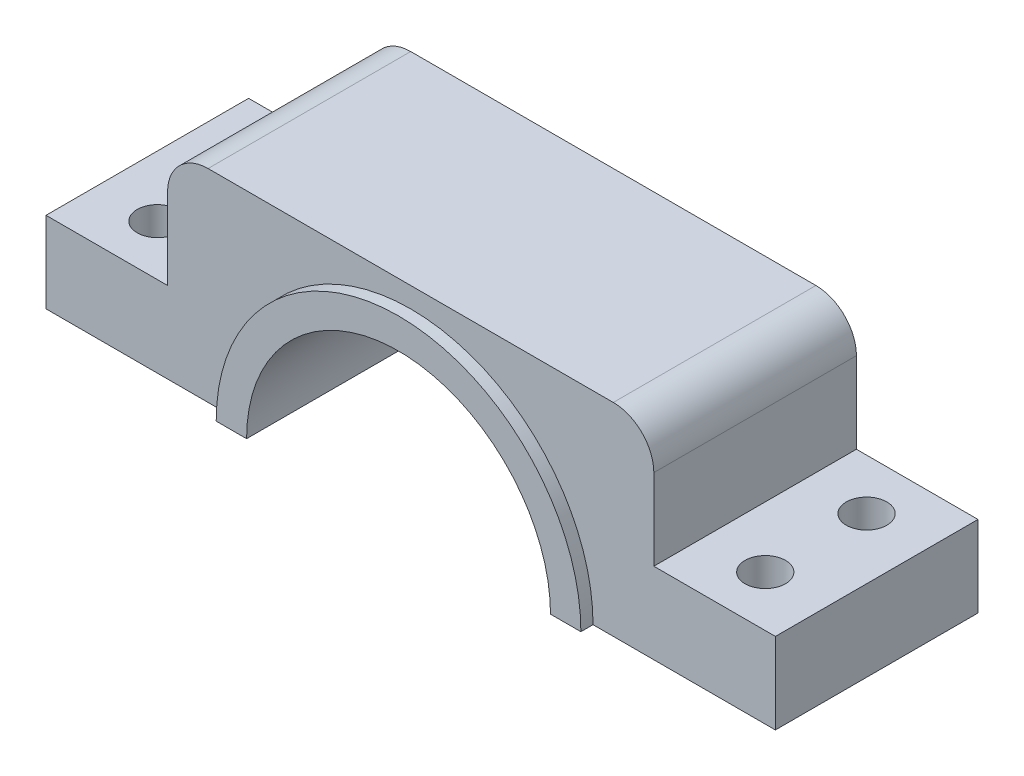
from build123d import *

# Parameters (mm, degrees)
SKETCH_2_W          = 120
SKETCH_2_H          = 50
EXTRUDE_1_DEPTH     = 50
SKETCH_3_R          = 37.5
CUT_EXTRUDE_1_DEPTH = 139
FILLET_1_R          = 10
SKETCH_4_W          = 30
SKETCH_4_H          = 50
EXTRUDE_2_DEPTH     = 20
EXTRUDE_START       = 3
EXTRUDE_3_DEPTH     = 3
SKETCH_6_R          = 5
CUT_EXTRUDE_2_DEPTH = 38


with BuildPart() as part:
    # 草图2 → 凸台-拉伸1 (new body)
    with BuildSketch(Plane(origin=(0, 0, 0), x_dir=(1, 0, 0), z_dir=(0, 1, 0))):
        Rectangle(SKETCH_2_W, SKETCH_2_H)
    extrude(amount=EXTRUDE_1_DEPTH)

    # 草图3 → 切除-拉伸1 (cut)
    with BuildSketch(Plane.XY.offset(25)):
        Circle(SKETCH_3_R)
    extrude(amount=-CUT_EXTRUDE_1_DEPTH, mode=Mode.SUBTRACT)

    # 圆角1
    fillet_1_edges = [part.edges().sort_by_distance(p)[0] for p in [
        (60, 50, 0),
        (-60, 50, 0),
    ]]
    fillet(fillet_1_edges, radius=FILLET_1_R)

    # 草图4 → 凸台-拉伸2 (add)
    with BuildSketch(Plane.XZ):
        with Locations((-75, 0)):
            Rectangle(SKETCH_4_W, SKETCH_4_H)
        with Locations((75, 0)):
            Rectangle(SKETCH_4_W, SKETCH_4_H)
    extrude(amount=-EXTRUDE_2_DEPTH)

    # 草图5 → 凸台-拉伸3 (add)
    with BuildSketch(Plane.XY.offset(25).offset(EXTRUDE_START)):
        with BuildLine():
            Line((-45, 0), (-37.5, 0))
            ThreePointArc((-37.5, 0), (0, 37.5), (37.5, 0))
            Line((37.5, 0), (45, 0))
            ThreePointArc((45, 0), (0, 45), (-45, 0))
        make_face()
    extrude_3 = extrude(amount=-EXTRUDE_3_DEPTH)

    # 镜向1: 凸台-拉伸3 across plane
    add(extrude_3.mirror(Plane.XY))

    # 草图6 → 切除-拉伸2 (cut)
    with BuildSketch(Plane(origin=(0, 20, 0), x_dir=(1, 0, 0), z_dir=(0, 1, 0))):
        with Locations(Location((-75, 12.5, 0), (0, 0, 270))):
            Circle(SKETCH_6_R)
        with Locations(Location((-75, -12.5, 0), (0, 0, 270))):
            Circle(SKETCH_6_R)
        with Locations(Location((75, -12.5, 0), (0, 0, 90))):
            Circle(SKETCH_6_R)
        with Locations(Location((75, 12.5, 0), (0, 0, 90))):
            Circle(SKETCH_6_R)
    extrude(amount=-CUT_EXTRUDE_2_DEPTH, mode=Mode.SUBTRACT)


solid = part.part
